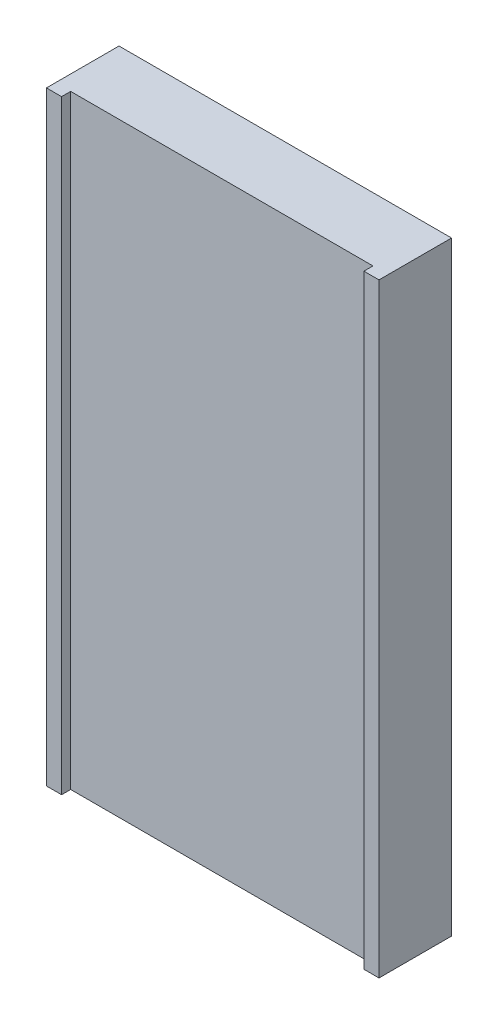
from build123d import *

# Parameters (mm, degrees)
SKETCH_1_W          = 55
SKETCH_1_H          = 100
EXTRUDE_1_DEPTH     = 12
SKETCH_2_W          = 50
SKETCH_2_H          = 100
CUT_EXTRUDE_1_DEPTH = 1.5


with BuildPart() as part:
    # 草图1 → 凸台-拉伸1 (new body)
    with BuildSketch(Plane.XY):
        Rectangle(SKETCH_1_W, SKETCH_1_H)
    extrude(amount=EXTRUDE_1_DEPTH)

    # 草图2 → 切除-拉伸1 (cut)
    with BuildSketch(Plane.XY.offset(12)):
        Rectangle(SKETCH_2_W, SKETCH_2_H)
    extrude(amount=-CUT_EXTRUDE_1_DEPTH, mode=Mode.SUBTRACT)


solid = part.part
